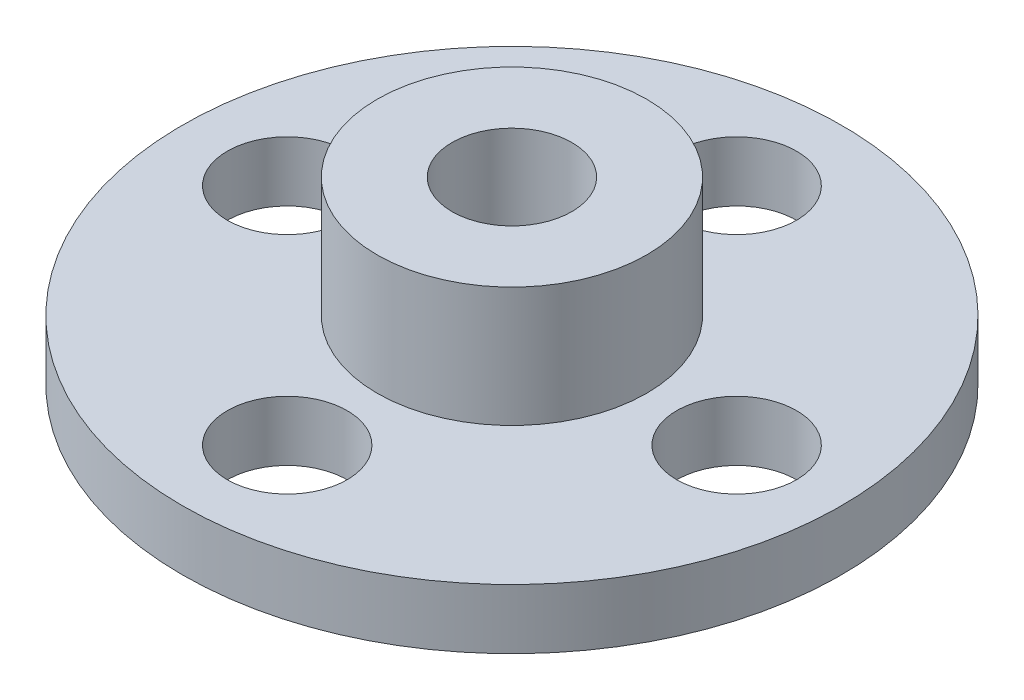
from build123d import *

# Parameters (mm, degrees)
SKETCH_1_R               = 11
SKETCH_1_R_2             = 2
EXTRUDE_1_DEPTH          = 2
SKETCH_2_R               = 4.5
EXTRUDE_2_DEPTH          = 4
CUT_EXTRUDE_1_DEPTH      = 17.673332001
CUT_EXTRUDE_1_DEPTH_BACK = 17.673332001
SKETCH_3_R               = 2


with BuildPart() as part:
    # 草图1 → 凸台-拉伸1 (new body)
    with BuildSketch(Plane(origin=(0, 0, 0), x_dir=(1, 0, 0), z_dir=(0, 1, 0))):
        with Locations(Location((0, 0, 0), (0, 0, 270))):
            Circle(SKETCH_1_R)
        with Locations(Location((0, 7.5, 0), (0, 0, 270))):
            Circle(SKETCH_1_R_2, mode=Mode.SUBTRACT)
        with Locations(Location((7.5, 0, 0), (0, 0, 270))):
            Circle(SKETCH_1_R_2, mode=Mode.SUBTRACT)
        with Locations(Location((0, -7.5, 0), (0, 0, 270))):
            Circle(SKETCH_1_R_2, mode=Mode.SUBTRACT)
        with Locations(Location((-7.5, 0, 0), (0, 0, 270))):
            Circle(SKETCH_1_R_2, mode=Mode.SUBTRACT)
    extrude(amount=EXTRUDE_1_DEPTH)

    # 草图2 → 凸台-拉伸2 (add)
    with BuildSketch(Plane(origin=(0, 2, 0), x_dir=(1, 0, 0), z_dir=(0, 1, 0))):
        with Locations(Location((0, 0, 0), (0, 0, 270))):
            Circle(SKETCH_2_R)
    extrude(amount=EXTRUDE_2_DEPTH)

    # 草图3 → 切除-拉伸1 (cut, two sides: drawn at the far end of the back side and taken through both)
    with BuildSketch(Plane(origin=(0, 6, 0), x_dir=(1, 0, 0), z_dir=(0, 1, 0)).offset(-CUT_EXTRUDE_1_DEPTH_BACK)):
        with Locations(Location((0, 0, 0), (0, 0, 270))):
            Circle(SKETCH_3_R)
    extrude(amount=CUT_EXTRUDE_1_DEPTH + CUT_EXTRUDE_1_DEPTH_BACK, mode=Mode.SUBTRACT)


solid = part.part
